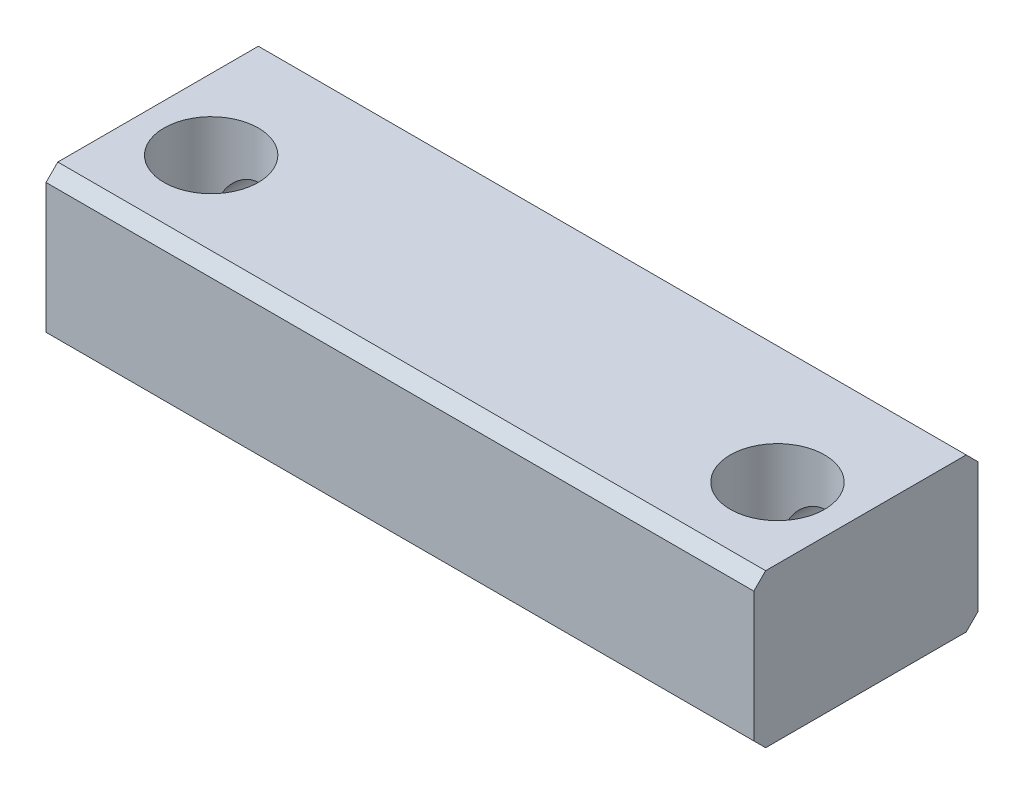
from build123d import *

# Parameters (mm, degrees)
SKETCH1_W              = 30
SKETCH1_H              = 6.5
BOSS_EXTRUDE1_DEPTH    = 9.5
SKETCH2_R              = 2
CUT_EXTRUDE1_DEPTH     = 19.907670401
M3_TAPPED_HOLE1_REACH  = 20.05
M3_TAPPED_HOLE1_BORE_R = 1.25
CHAMFER1_SIZE          = 0.5


with BuildPart() as part:
    # Sketch1 → Boss-Extrude1 (new body)
    with BuildSketch(Plane.XY):
        Rectangle(SKETCH1_W, SKETCH1_H)
    extrude(amount=BOSS_EXTRUDE1_DEPTH)

    # Sketch2 → Cut-Extrude1 (cut, through all)
    with BuildSketch(Plane(origin=(0, 3.25, 0), x_dir=(1, 0, 0), z_dir=(0, 1, 0))):
        with Locations(Location((-12, -5.5, 0), (0, 0, 180))):
            Circle(SKETCH2_R)
        with Locations(Location((12, -5.5, 0), (0, 0, 180))):
            Circle(SKETCH2_R)
    extrude(amount=-CUT_EXTRUDE1_DEPTH, mode=Mode.SUBTRACT)

    # M3 Tapped Hole1 bore → M3 Tapped Hole1 (cut, up to next)
    with BuildSketch(Plane(origin=(0, 0, 0), x_dir=(-1, 0, 0), z_dir=(0, 0, -1)), mode=Mode.PRIVATE) as m3_tapped_hole1_sk1:
        with Locations((12, 0)):
            Circle(M3_TAPPED_HOLE1_BORE_R)
    m3_tapped_hole1_tool1 = extrude(m3_tapped_hole1_sk1.sketch, amount=-M3_TAPPED_HOLE1_REACH, mode=Mode.PRIVATE) & part.part
    # M3 Tapped Hole1 bore → M3 Tapped Hole1 (cut, up to next)
    with BuildSketch(Plane(origin=(0, 0, 0), x_dir=(-1, 0, 0), z_dir=(0, 0, -1)), mode=Mode.PRIVATE) as m3_tapped_hole1_sk2:
        with Locations((-12, 0)):
            Circle(M3_TAPPED_HOLE1_BORE_R)
    m3_tapped_hole1_tool2 = extrude(m3_tapped_hole1_sk2.sketch, amount=-M3_TAPPED_HOLE1_REACH, mode=Mode.PRIVATE) & part.part
    add(m3_tapped_hole1_tool1.solids().sort_by_distance((-12, 0, 0))[0], mode=Mode.SUBTRACT)
    add(m3_tapped_hole1_tool2.solids().sort_by_distance((12, 0, 0))[0], mode=Mode.SUBTRACT)

    # Chamfer1
    chamfer1_edges = [part.edges().sort_by_distance(p)[0] for p in [
        (0, 3.25, 9.5),
        (0, 3.25, 0),
        (0, -3.25, 0),
        (0, -3.25, 9.5),
    ]]
    chamfer(chamfer1_edges, length=CHAMFER1_SIZE)


solid = part.part
